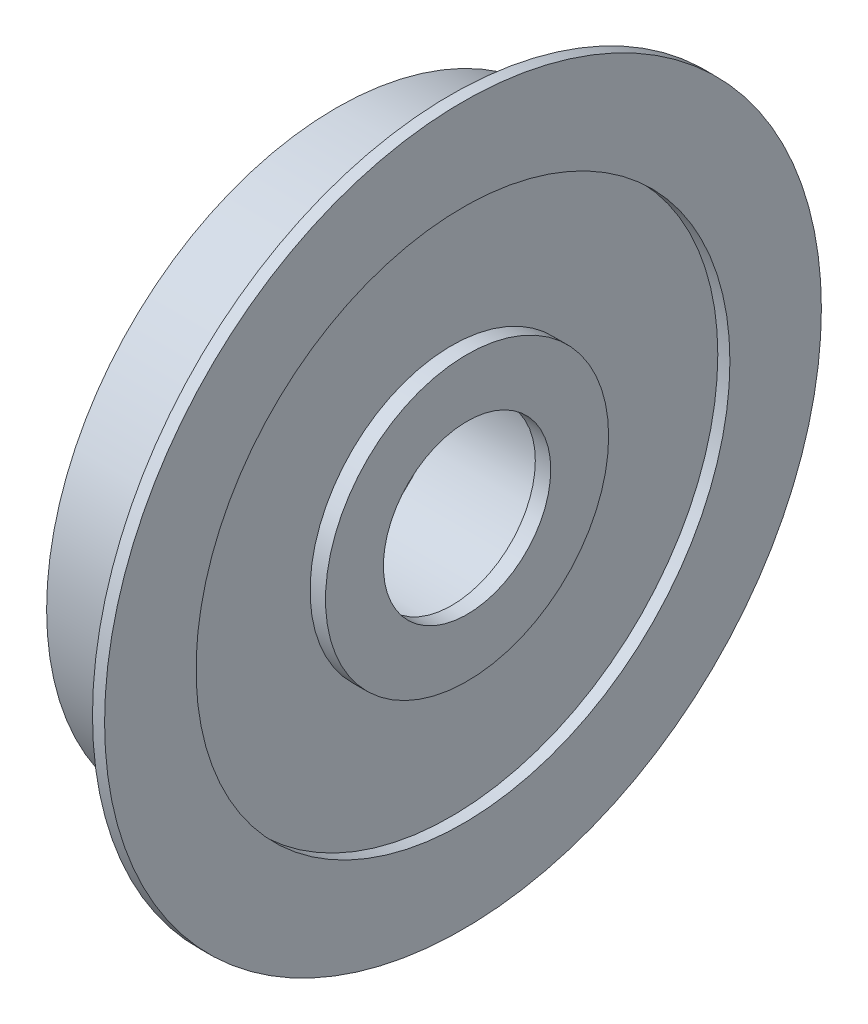
SolidWorks part; units mm, degrees
ref_plane "Front Plane" through (0, 0, 0) normal (0, 0, 1) x (1, 0, 0)
ref_plane "Top Plane" through (0, 0, 0) normal (0, 1, 0) x (1, 0, 0)
ref_plane "Right Plane" through (0, 0, 0) normal (1, 0, 0) x (0, 0, -1)
sketch "Sketch1" plane through (0, 0, 0) normal (0, 0, 1) x (1, 0, 0)
  line L0 (108, 30.3761) -> (108, 24.55)
  line L1 (108, -31.426) -> (108, 31.426) construction
  line L2 (108, -24.55) -> (108, 24.55) construction
  line L3 (108, 24.55) -> (98.2863, 24.55)
  line L4 (98.2863, -24.55) -> (98.2863, 24.55) construction
  line L5 (98.2863, 24.55) -> (98.2863, 8.6596)
  line L6 (98.2863, -8.6596) -> (98.2863, 8.6596) construction
  line L7 (98.2863, -10.6596) -> (98.2863, 10.6596) construction
  line L8 (98.2863, 8.6596) -> (108, 8.6596)
  line L9 (108, -8.6596) -> (108, 8.6596) construction
  line L10 (108, 8.6596) -> (108, 22.6232)
  line L11 (108, 22.6232) -> (109.0254, 22.6232)
  line L12 (109.0254, 22.6232) -> (109.0254, 30.3761)
  line L13 (109.0254, 30.3761) -> (108, 30.3761)
  line L14 (0, 0) -> (-9.1422, 0) construction
  line L15 (108.0647, 7.0916) -> (109.3716, 7.0916)
  line L16 (108.0647, 7.0916) -> (108.0647, 11.9988)
  line L17 (108.0647, 11.9988) -> (109.3716, 11.9988)
  line L18 (109.3716, 7.0916) -> (109.3716, 11.9988)
  spline S0 degree 3 poles (109.5, 21.6369) (109.4368, 21.6666) (109.3761, 21.714) (109.2631, 21.843) (109.2104, 21.9261) (109.1222, 22.1199) (109.0851, 22.2347) (109.0352, 22.4801) (109.0215, 22.6143) (109.0214, 22.8852) (109.0347, 23.0169) (109.0849, 23.2648) (109.1214, 23.3781) (109.2546, 23.6715) (109.3745, 23.804) (109.5, 23.8631) knots 0 0 0 0 0.125 0.125 0.25 0.25 0.375 0.375 0.5 0.5 0.625 0.625 0.75 0.75 1 1 1 1 construction
revolve "Revolve1" add sketch "Sketch1" angle 360 about L14
